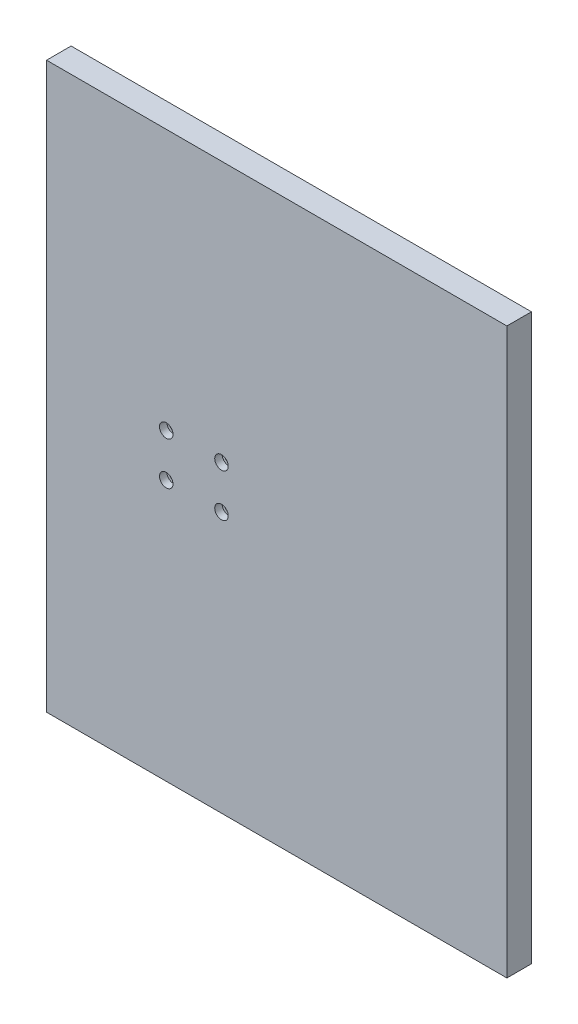
from build123d import *

# Parameters (mm, degrees)
SKETCH1_W                               = 375
SKETCH1_H                               = 460
BOSS_EXTRUDE1_DEPTH                     = 20
CBORE_FOR_M6_HEX_HEAD_BOLT1_D           = 6.6
CBORE_FOR_M6_HEX_HEAD_BOLT1_CBORE_D     = 11
CBORE_FOR_M6_HEX_HEAD_BOLT1_CBORE_DEPTH = 6


with BuildPart() as part:
    # Sketch1 → Boss-Extrude1 (new body)
    with BuildSketch(Plane.XY):
        with Locations((67.5, 230)):
            Rectangle(SKETCH1_W, SKETCH1_H)
    extrude(amount=BOSS_EXTRUDE1_DEPTH)

    # CBORE for M6 Hex Head Bolt1 (through all)
    with Locations(Plane.XY.offset(20)):
        with Locations((-22.5, 247.5), (22.5, 247.5), (22.5, 212.5), (-22.5, 212.5)):
            CounterBoreHole(CBORE_FOR_M6_HEX_HEAD_BOLT1_D / 2, CBORE_FOR_M6_HEX_HEAD_BOLT1_CBORE_D / 2, CBORE_FOR_M6_HEX_HEAD_BOLT1_CBORE_DEPTH)


solid = part.part
